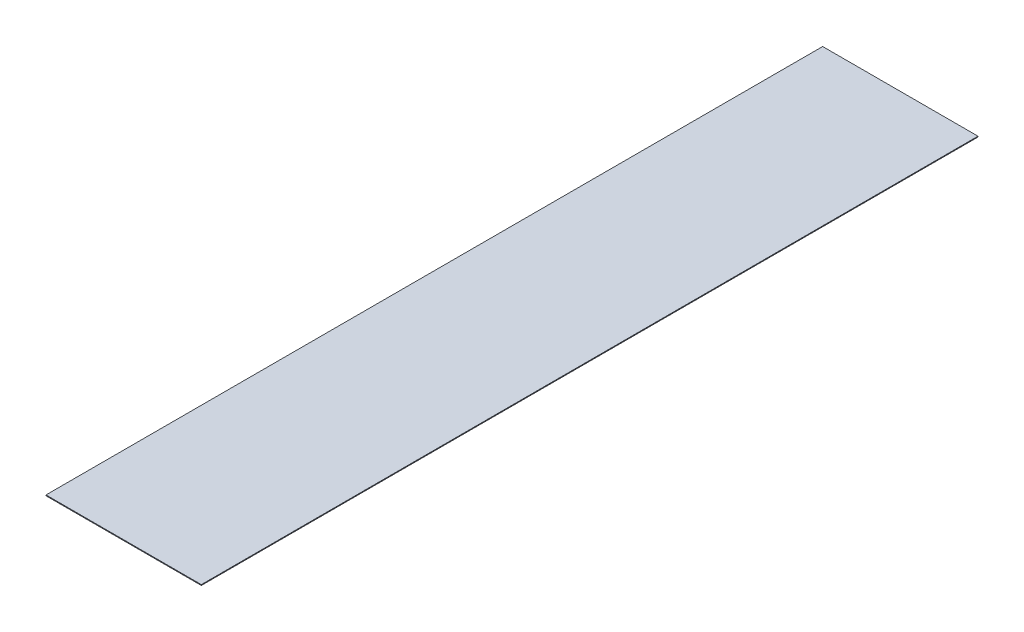
SolidWorks part; units mm, degrees
ref_plane "Front Plane" through (0, 0, 0) normal (0, 0, 1) x (1, 0, 0)
ref_plane "Top Plane" through (0, 0, 0) normal (0, 1, 0) x (1, 0, 0)
ref_plane "Right Plane" through (0, 0, 0) normal (1, 0, 0) x (0, 0, -1)
sketch "Sketch1" plane through (0, 0, 0) normal (0, 1, 0) x (1, 0, 0)
  line L1 (-100, -500) -> (100, -500)
  line L2 (-100, -500) -> (-100, 500)
  line L3 (-100, 500) -> (100, 500)
  line L4 (100, -500) -> (100, 500)
  line L5 (-100, -500) -> (100, 500) construction
  line L6 (-100, 500) -> (100, -500) construction
  point P0 (0, 0)
  dimension "D1" = 200
  dimension "D2" = 1000
extrude "Boss-Extrude1" add sketch "Sketch1" along normal blind 1
